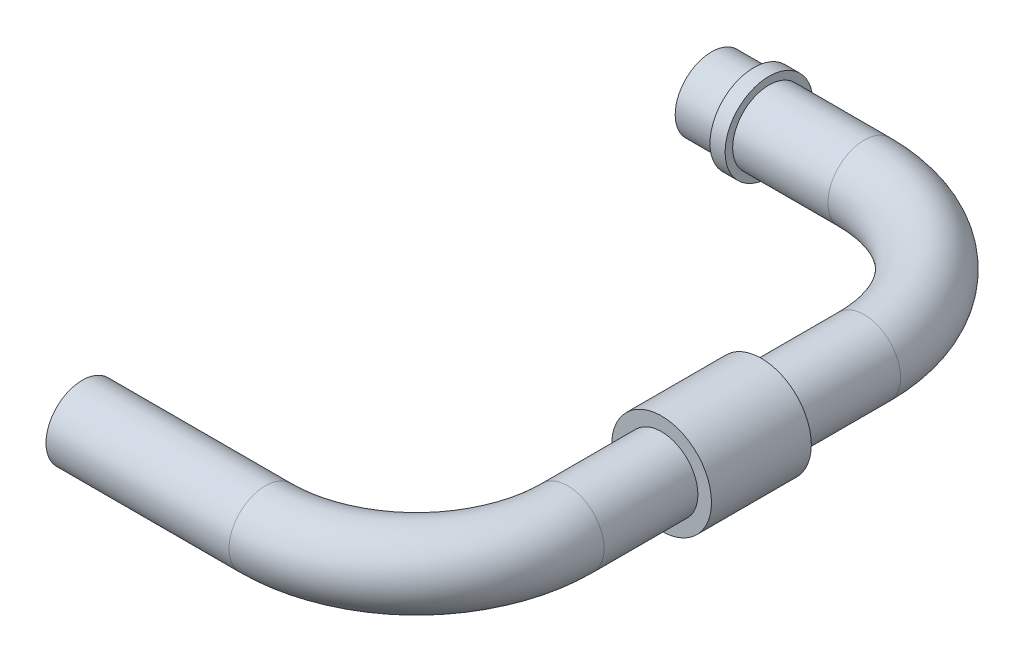
from build123d import *

# Parameters (mm, degrees)
SWEEP_1_PROFILE_R = 12
EXTRUDE_START     = -14
SKETCH_14_R       = 14.5
EXTRUDE_1_DEPTH   = 5
SKETCH_16_R       = 16.5
EXTRUDE_2_DEPTH   = 16.5


with BuildPart() as part:
    # 扫描1: sweep along a path in 草图1
    with BuildLine(Plane(origin=(0, 0, 0), x_dir=(1, 0, 0), z_dir=(0, 1, 0))) as sweep_1_path:
        Line((0, 0), (60.5, 0))
        ThreePointArc((60.5, 0), (95.855339059, 14.644660941), (110.5, 50))
        Line((110.5, 50), (110.5, 148))
        ThreePointArc((110.5, 148), (95.855339059, 183.355339059), (60.5, 198))
        Line((60.5, 198), (10, 198))
    # 扫描1 profile (on start of the path) → 扫描1 (sweep)
    with BuildSketch(Plane(origin=(0, 0, 0), x_dir=(0, 0, 1), z_dir=(1, 0, 0))):
        Circle(SWEEP_1_PROFILE_R)
    sweep(path=sweep_1_path.line)

    # 草图14 → 凸台-拉伸1 (add)
    with BuildSketch(Plane.ZY.offset(-10).offset(EXTRUDE_START)):
        with Locations((-198, 0)):
            Circle(SKETCH_14_R)
    extrude(amount=-EXTRUDE_1_DEPTH)

    # 草图16 → 凸台-拉伸2 (add, symmetric)
    with BuildSketch(Plane.XY.offset(-97.5)):
        with Locations((110.5, 0)):
            Circle(SKETCH_16_R)
    extrude(amount=EXTRUDE_2_DEPTH, both=True)


solid = part.part
